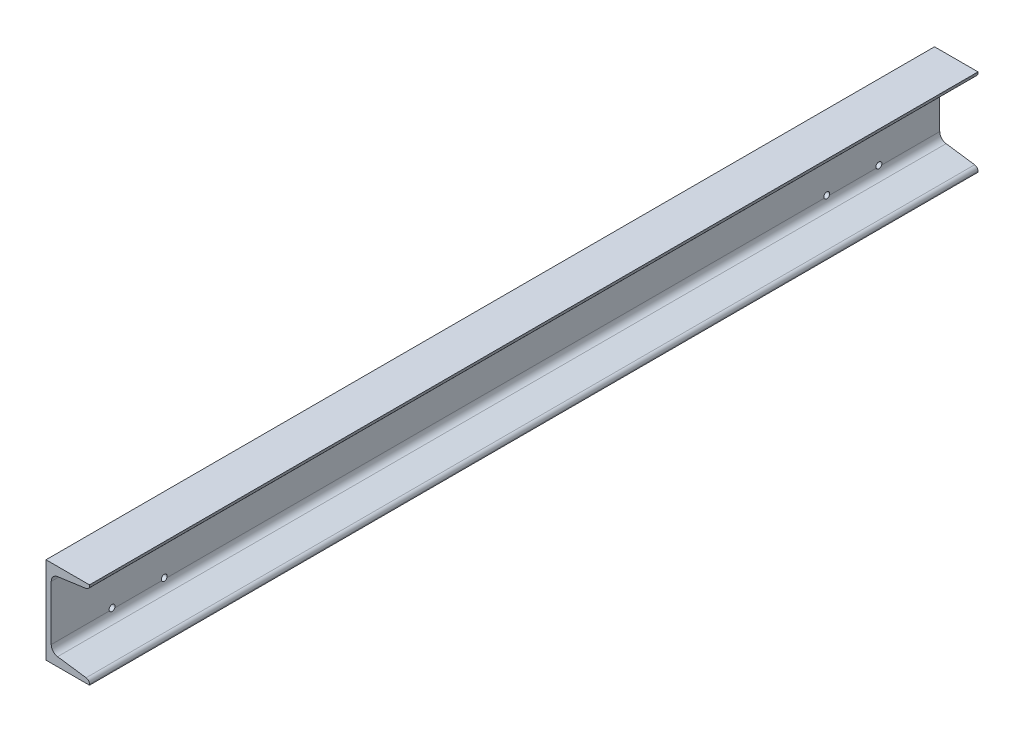
from build123d import *

# Parameters (mm, degrees)
BOSS_EXTRUDE1_DEPTH   = 1022
M8_TAPPED_HOLE1_D     = 6.8
M8_TAPPED_HOLE1_DEPTH = 19.75
M8_TAPPED_HOLE1_TIP   = 2.042926105


with BuildPart() as part:
    # Sketch1 → Boss-Extrude1 (new body)
    with BuildSketch(Plane.XY):
        with BuildLine():
            Line((0, 0), (-50, 0))
            Line((-50, 0), (-50, -100))
            Line((-50, -100), (0, -100))
            Line((0, -100), (0, -98.925311188))
            ThreePointArc((0, -98.925311188), (-1.103806889, -95.973045557), (-3.873721046, -94.469104878))
            Line((-3.873721046, -94.469104878), (-36.682971358, -89.858065454))
            ThreePointArc((-36.682971358, -89.858065454), (-41.915031432, -87.017288616), (-44, -81.440786869))
            Line((-44, -81.440786869), (-44, -18.559213131))
            ThreePointArc((-44, -18.559213131), (-41.915031432, -12.982711384), (-36.682971358, -10.141934546))
            Line((-36.682971358, -10.141934546), (-3.873721046, -5.530895122))
            ThreePointArc((-3.873721046, -5.530895122), (-1.103806889, -4.026954443), (0, -1.074688812))
            Line((0, -1.074688812), (0, 0))
        make_face()
    extrude(amount=BOSS_EXTRUDE1_DEPTH)

    # M8 Tapped Hole1
    with Locations(Plane.ZY.offset(50)):
        with Locations((70, -20), (130, -20), (130, -80), (70, -80), (892, -20), (952, -20), (952, -80), (892, -80)):
            Hole(M8_TAPPED_HOLE1_D / 2, depth=M8_TAPPED_HOLE1_DEPTH)
            with Locations((0, 0, -(M8_TAPPED_HOLE1_DEPTH + M8_TAPPED_HOLE1_TIP / 2))):  # 118° drill point
                Cone(0, M8_TAPPED_HOLE1_D / 2, M8_TAPPED_HOLE1_TIP, mode=Mode.SUBTRACT)


solid = part.part
